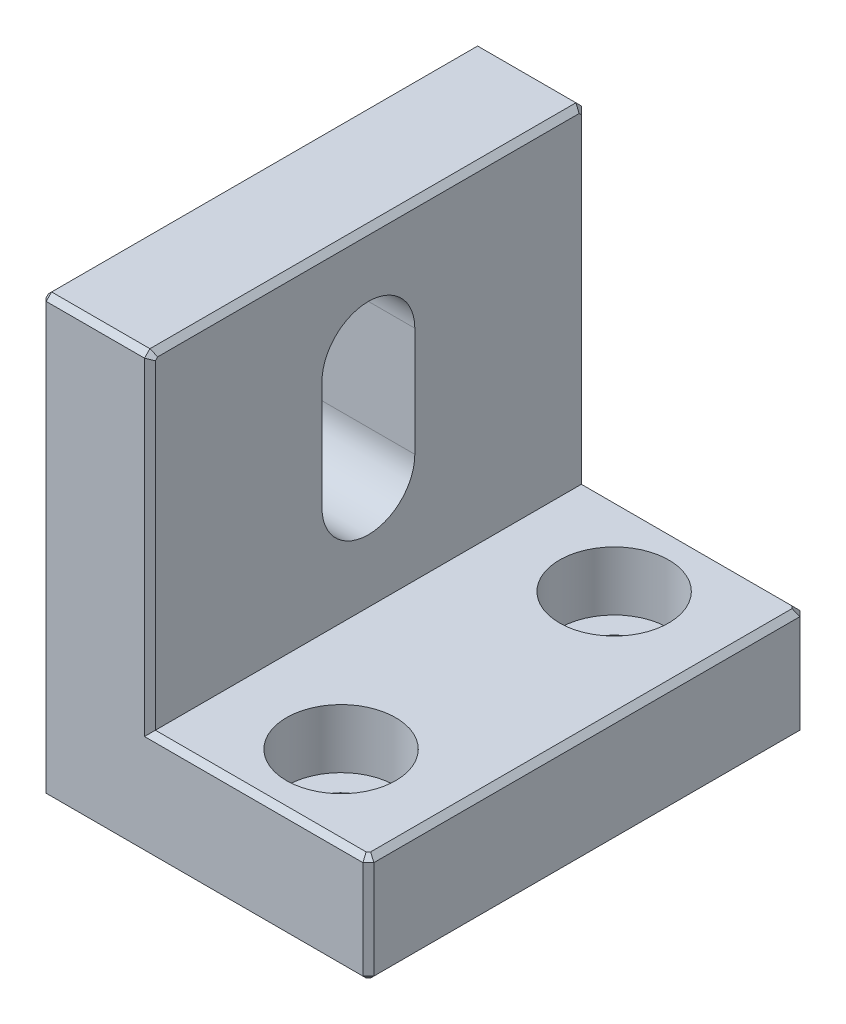
from build123d import *

# Parameters (mm, degrees)
SKETCH_1_W                   = 30
SKETCH_1_H                   = 40
EXTRUDE_1_DEPTH              = 10
SKETCH_2_W                   = 40
SKETCH_2_H                   = 40
EXTRUDE_2_DEPTH              = 10
HOLE_WIZARD_M5_1_D           = 5.5
HOLE_WIZARD_M5_1_CBORE_D     = 10
HOLE_WIZARD_M5_1_CBORE_DEPTH = 5.4
CHAMFER_1_SIZE               = 0.5
CUT_EXTRUDE_1_DEPTH          = 49.989794856
CHAMFER_2_SIZE               = 0.5
CHAMFER_3_SIZE               = 0.5


with BuildPart() as part:
    # 草图1 → 凸台-拉伸1 (new body)
    with BuildSketch(Plane(origin=(0, 0, 0), x_dir=(1, 0, 0), z_dir=(0, 1, 0))):
        Rectangle(SKETCH_1_W, SKETCH_1_H)
    extrude(amount=EXTRUDE_1_DEPTH)

    # 草图2 → 凸台-拉伸2 (add)
    with BuildSketch(Plane.ZY.offset(15)):
        with Locations((0, 20)):
            Rectangle(SKETCH_2_W, SKETCH_2_H)
    extrude(amount=-EXTRUDE_2_DEPTH)

    # M5 六角凹头螺钉的柱形沉头孔1 (through all)
    with Locations(Plane(origin=(0, 10, 0), x_dir=(1, 0, 0), z_dir=(0, 1, 0))):
        with Locations((5, -12.5), (5, 12.5)):
            CounterBoreHole(HOLE_WIZARD_M5_1_D / 2, HOLE_WIZARD_M5_1_CBORE_D / 2, HOLE_WIZARD_M5_1_CBORE_DEPTH)

    # 倒角1
    chamfer_1_edges = [part.edges().sort_by_distance(p)[0] for p in [
        (15, 5, 20),
        (15, 5, -20),
    ]]
    chamfer(chamfer_1_edges, length=CHAMFER_1_SIZE)

    # 草图5 → 切除-拉伸1 (cut, through all)
    with BuildSketch(Plane(origin=(-5, 0, 0), x_dir=(0, 0, -1), z_dir=(1, 0, 0))):
        with BuildLine():
            Line((4.25, 30), (4.25, 20))
            ThreePointArc((4.25, 20), (0, 15.75), (-4.25, 20))
            Line((-4.25, 20), (-4.25, 30))
            ThreePointArc((-4.25, 30), (0, 34.25), (4.25, 30))
        make_face()
    extrude(amount=-CUT_EXTRUDE_1_DEPTH, mode=Mode.SUBTRACT)

    # 倒角2
    chamfer_2_edges = [part.edges().sort_by_distance(p)[0] for p in [
        (-10, 40, -20),
        (-10, 40, 20),
    ]]
    chamfer(chamfer_2_edges, length=CHAMFER_2_SIZE)

    # 倒角3
    chamfer_3_edges = [part.edges().sort_by_distance(p)[0] for p in [
        (4.75, 10, 20),
        (-5, 24.75, 20),
        (-0.25, 0, 20),
        (-15, 0, 0),
        (-0.25, 0, -20),
        (4.75, 10, -20),
        (15, 0, 0),
        (14.75, 0, 19.75),
        (14.75, 0, -19.75),
        (15, 10, 0),
        (14.75, 10, 19.75),
        (14.75, 10, -19.75),
        (-15, 19.75, 20),
        (-15, 40, 0),
        (-15, 19.75, -20),
        (-15, 39.75, -19.75),
        (-15, 39.75, 19.75),
        (-5, 40, 0),
        (-5, 24.75, -20),
        (-5, 39.75, -19.75),
        (-5, 39.75, 19.75),
    ]]
    chamfer(chamfer_3_edges, length=CHAMFER_3_SIZE)


solid = part.part
